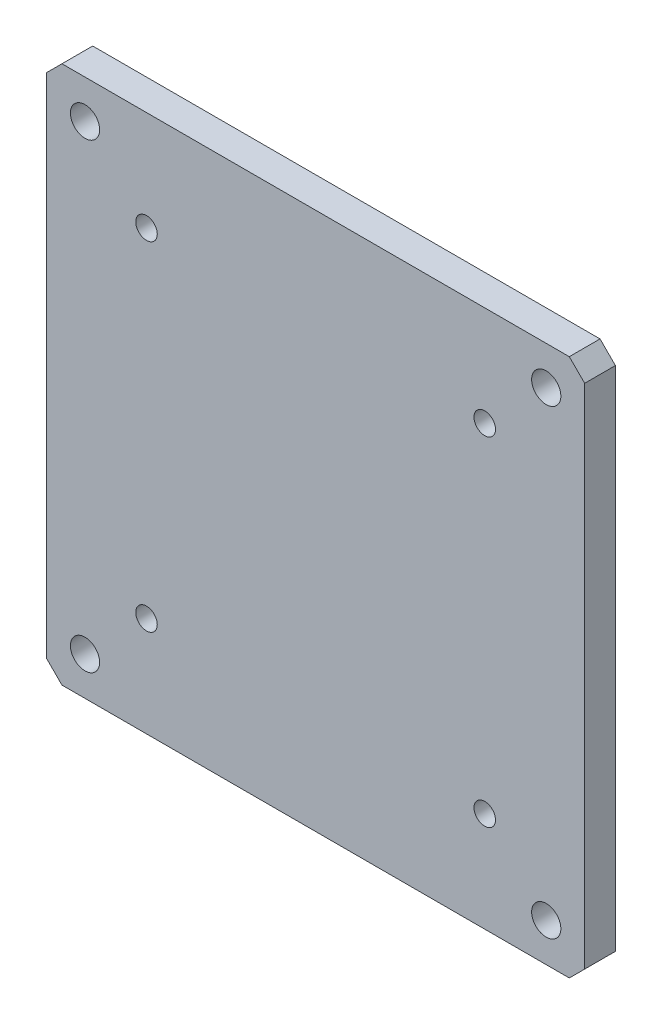
SolidWorks part; units mm, degrees
material "Q235A"
ref_plane "前视基准面" through (0, 0, 0) normal (0, 0, 1) x (1, 0, 0)
ref_plane "上视基准面" through (0, 0, 0) normal (0, 1, 0) x (1, 0, 0)
ref_plane "右视基准面" through (0, 0, 0) normal (1, 0, 0) x (0, 0, -1)
sketch "草图1" plane through (0, 0, 0) normal (0, 0, 1) x (1, 0, 0)
  line L1 (-175, 175) -> (175, 175)
  line L2 (-175, 175) -> (-175, -175)
  line L3 (-175, -175) -> (175, -175)
  line L4 (175, 175) -> (175, -175)
  line L5 (0, -175) -> (0, 175) construction
  line L6 (-175, 0) -> (175, 0) construction
  point P0 (0, 0)
  dimension "D1" = 350
  dimension "D2" = 350
extrude "凸台-拉伸1" add sketch "草图1" along normal blind 20
hole_wizard "M16 螺纹孔1" positions "草图2" profile "草图3" tap size "M16" standard "GB"
sketch "草图2" plane through (0, 0, 20) normal (0, 0, 1) x (1, 0, 0)
  line L1 (-110, -110) -> (110, -110) construction
  line L2 (-110, -110) -> (-110, 110) construction
  line L3 (-110, 110) -> (110, 110) construction
  line L4 (110, -110) -> (110, 110) construction
  line L5 (0, 110) -> (0, -110) construction
  line L6 (-110, 0) -> (110, 0) construction
  point P2 (110, 110)
  point P237 (-110, -110)
  point P238 (-110, 110)
  point P254 (110, -110)
  dimension "D1" = 220
  dimension "D2" = 220
sketch "草图3" plane through (110, 110, 20) normal (1, 0, 0) x (0, -1, 0)
  line L0 (0, 0) -> (0, 46.206)
  line L1 (0, 46.206) -> (7, 42)
  line L2 (7, 42) -> (7, 0)
  line L5 (7, 0) -> (0, 0)
  line L10 (0, 46.206) -> (-7, 42) construction
  line L11 (0, -6.35) -> (0, 107.95) construction
  dimension "螺纹孔钻头直径" = 14
  dimension "螺纹孔钻头深度" = 42
  dimension "导头角度" = 118
cosmetic thread "孔螺蚊线1" parameters "D1"=20, "D2"=16
cosmetic thread "孔螺蚊线4" parameters "D1"=20, "D2"=16
cosmetic thread "孔螺蚊线5" parameters "D1"=20, "D2"=16
cosmetic thread "孔螺蚊线6" parameters "D1"=20, "D2"=16
hole_wizard "Ø19.0 (19) 直径孔1" positions "草图4" profile "草图5" hole size "Ø19.0" standard "GB"
sketch "草图4" plane through (0, 0, 20) normal (0, 0, 1) x (1, 0, 0)
  line L1 (-150, -150) -> (150, -150) construction
  line L2 (-150, -150) -> (-150, 150) construction
  line L3 (-150, 150) -> (150, 150) construction
  line L4 (150, -150) -> (150, 150) construction
  line L5 (0, 150) -> (0, -150) construction
  line L6 (-150, 0) -> (150, 0) construction
  point P2 (150, 150)
  point P291 (-150, -150)
  point P292 (-150, 150)
  point P293 (150, -150)
  dimension "D1" = 300
  dimension "D2" = 300
sketch "草图5" plane through (150, 150, 20) normal (1, 0, 0) x (0, -1, 0)
  line L0 (0, 0) -> (0, 30.7082)
  line L1 (0, 30.7082) -> (9.5, 25)
  line L2 (9.5, 25) -> (9.5, 0)
  line L5 (9.5, 0) -> (0, 0)
  line L10 (0, 30.7082) -> (-9.5, 25) construction
  line L11 (0, -6.35) -> (0, 107.95) construction
  dimension "孔直径" = 19
  dimension "孔深度" = 25
  dimension "导头角度" = 118
chamfer "倒角1" distance 10 angle 45 4 edges at (-175, -175, 10) (175, -175, 10) (175, 175, 10) (-175, 175, 10)
